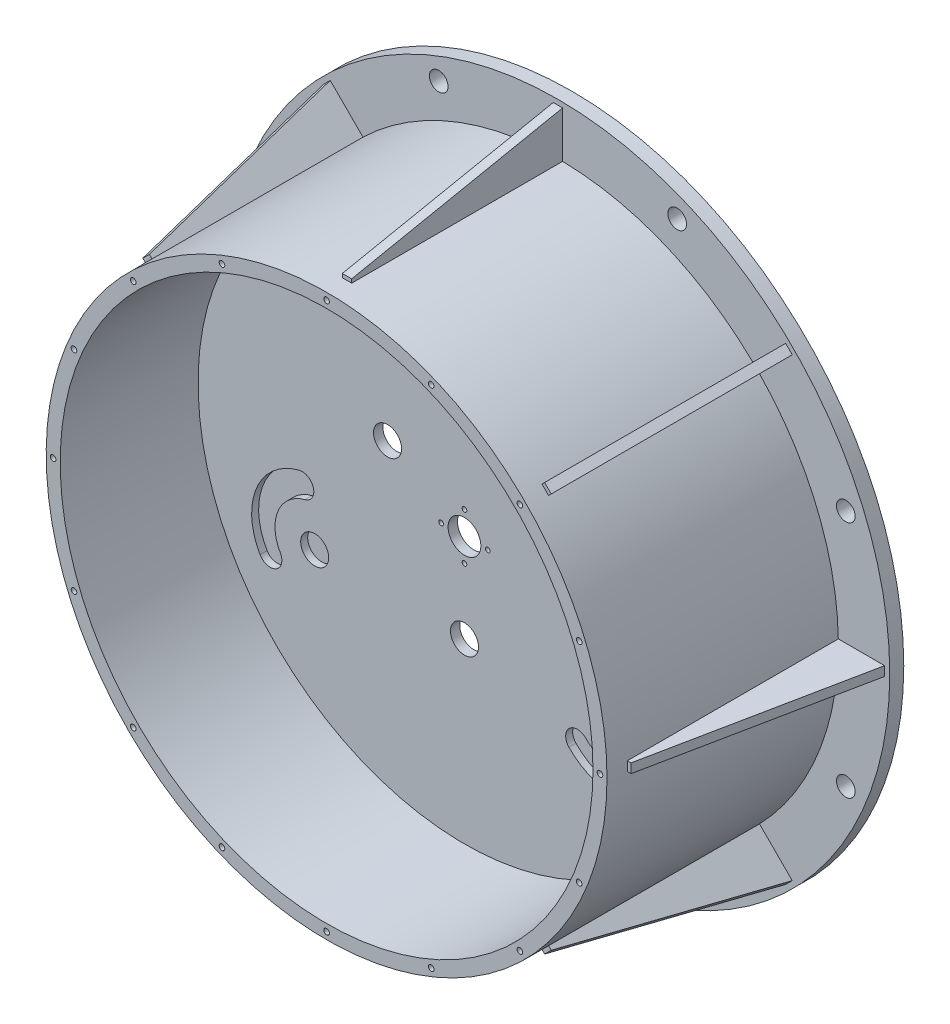
SolidWorks part; units mm, degrees
ref_plane "Front Plane" through (0, 0, 0) normal (0, 0, 1) x (1, 0, 0)
ref_plane "Top Plane" through (0, 0, 0) normal (0, 1, 0) x (1, 0, 0)
ref_plane "Right Plane" through (0, 0, 0) normal (1, 0, 0) x (0, 0, -1)
sketch "Sketch1" plane through (0, 0, 0) normal (0, 0, 1) x (1, 0, 0)
  circle A0 centre (0, 0) radius 600
  dimension "D1" = 1200
extrude "Boss-Extrude1" add sketch "Sketch1" along normal blind 20
sketch "Sketch2" plane through (0, 0, 0) normal (0, 0, -1) x (-1, 0, 0)
  circle A0 centre (0, 0) radius 35
  circle A1 centre (0, 0) radius 50 construction
  circle A2 centre (50, 0) radius 5
  circle A3 centre (0, -50) radius 5
  circle A4 centre (-50, 0) radius 5
  circle A5 centre (0, 50) radius 5
  point P15 (0, 0)
  dimension "D1" = 70
  dimension "D2" = 100
  dimension "D3" = 10
  dimension "D4" = 4
extrude "Cut-Extrude1" cut sketch "Sketch2" against normal through all
sketch "Sketch3" plane through (0, 0, 0) normal (0, 0, -1) x (-1, 0, 0)
  line L0 (0, 0) -> (0, -190) construction
  circle A0 centre (0, -190) radius 30
  dimension "D2" = 60
  dimension "D1" = 190
extrude "Cut-Extrude2" cut sketch "Sketch3" against normal through all
pattern_circular "CirPattern1" count 3 over 360 about axis through (0, 0, 0) along (0, 0, 1) of "Cut-Extrude2"
sketch "Sketch4" plane through (0, 0, 20) normal (0, 0, 1) x (1, 0, 0)
  circle A0 centre (0, 0) radius 600
  circle A1 centre (0, 0) radius 570
  dimension "D1" = 30
  dimension "D2" = 1200
extrude "Boss-Extrude2" add sketch "Sketch4" against normal blind 200
sketch "Sketch6" plane through (0, 0, 20) normal (0, 0, 1) x (1, 0, 0)
  line L0 (0, 0) -> (0, 550) construction
  circle A2 centre (0, 370) radius 30
  circle A3 centre (320.4294, -185) radius 30
  circle A4 centre (-320.4294, -185) radius 30
  arc A5 (96.3228, 316.8783) -> (-24.8381, 477.1591) centre (0, 370) ccw construction
  arc A10 (437.3428, -252.5) -> (394.0416, -227.5) centre (415.6922, -240) ccw
  arc A11 (259.4645, -244.2307) -> (394.0416, -227.5) centre (320.4294, -185) ccw
  arc A12 (259.4645, -244.2307) -> (223.6028, -279.0723) centre (241.5336, -261.6515) ccw
  arc A13 (223.6028, -279.0723) -> (437.3428, -252.5) centre (320.4294, -185) ccw
  arc A14 (-437.3428, -252.5) -> (-394.0416, -227.5) centre (-415.6922, -240) ccw
  arc A15 (-341.2422, -102.5875) -> (-394.0416, -227.5) centre (-320.4294, -185) ccw
  arc A16 (-341.2422, -102.5875) -> (-353.4851, -54.1095) centre (-347.3637, -78.3485) ccw
  arc A17 (-353.4851, -54.1095) -> (-437.3428, -252.5) centre (-320.4294, -185) ccw
  arc A30 (81.7778, 346.8182) -> (0, 455) centre (0, 370) ccw
  arc A31 (0, 505) -> (0, 455) centre (0, 480) ccw
  arc A32 (129.8823, 333.1818) -> (0, 505) centre (0, 370) ccw
  arc A33 (81.7778, 346.8182) -> (129.8823, 333.1818) centre (105.8301, 340) ccw
  point P11 (0, 0)
  point P37 (0, 0)
  dimension "D1" = 60
  dimension "D2" = 60
  dimension "D4" = 60
  dimension "D5" = 220
extrude "Cut-Extrude3" cut sketch "Sketch6" against normal blind 15
sketch "Sketch7" plane through (0, 0, 20) normal (0, 0, 1) x (1, 0, 0)
  circle A0 centre (0, 0) radius 600
  circle A1 centre (0, 0) radius 570
  dimension "D1" = 1200
  dimension "D2" = 30
extrude "Boss-Extrude3" add sketch "Sketch7" along normal blind 295
sketch "Sketch8" plane through (0, 0, -180) normal (0, 0, -1) x (-1, 0, 0)
  line L0 (0, 0) -> (710, 0) construction
  line L1 (0, 0) -> (615.9803, -255.1474) construction
  circle A0 centre (0, 0) radius 570
  circle A1 centre (0, 0) radius 710
  circle A2 centre (-615.9803, 255.1474) radius 20
  circle A3 centre (-255.1474, 615.9803) radius 20
  circle A4 centre (255.1474, 615.9803) radius 20
  circle A5 centre (615.9803, 255.1474) radius 20
  circle A6 centre (615.9803, -255.1474) radius 20
  circle A7 centre (255.1474, -615.9803) radius 20
  circle A8 centre (-255.1474, -615.9803) radius 20
  circle A9 centre (-615.9803, -255.1474) radius 20
  point P23 (0, 0)
  dimension "D1" = 1420
  dimension "D2" = 40
  dimension "D5" = 1140
  dimension "D4" = 22.5
  dimension "D3" = 8
extrude "Boss-Extrude4" add sketch "Sketch8" along normal blind 30
sketch "Sketch9" plane through (0, 0, 315) normal (0, 0, 1) x (1, 0, 0)
  circle A0 centre (0, 0) radius 585 construction
  circle A1 centre (585, 0) radius 6
  circle A2 centre (540.4695, -223.8698) radius 6
  circle A3 centre (413.6575, -413.6575) radius 6
  circle A4 centre (223.8698, -540.4695) radius 6
  circle A5 centre (0, -585) radius 6
  circle A6 centre (-223.8698, -540.4695) radius 6
  circle A7 centre (-413.6575, -413.6575) radius 6
  circle A8 centre (-540.4695, -223.8698) radius 6
  circle A9 centre (-585, 0) radius 6
  circle A10 centre (-540.4695, 223.8698) radius 6
  circle A11 centre (-413.6575, 413.6575) radius 6
  circle A12 centre (-223.8698, 540.4695) radius 6
  circle A13 centre (0, 585) radius 6
  circle A14 centre (223.8698, 540.4695) radius 6
  circle A15 centre (413.6575, 413.6575) radius 6
  circle A16 centre (540.4695, 223.8698) radius 6
  point P38 (0, 0)
  dimension "D1" = 12
  dimension "D3" = 1170
  dimension "D2" = 16
extrude "Cut-Extrude4" cut sketch "Sketch9" against normal blind 30
sketch "Sketch10" plane through (0, 0, 0) normal (0, 1, 0) x (1, 0, 0)
  line L1 (-600, 180) -> (600, 180) construction
  line L2 (-594.3176, 180) -> (-594.3176, -271.3296)
  line L4 (-607.9361, -271.3296) -> (-698.9937, 180)
  line L5 (-710, 180) -> (710, 180) construction
  line L6 (-698.9937, 180) -> (-594.3176, 180)
  line L7 (-594.3176, -271.3296) -> (-607.9361, -271.3296)
extrude "Boss-Extrude5" add sketch "Sketch10" along normal mid plane 20
pattern_circular "CirPattern2" count 8 over 360 about axis through (0, 0, 0) along (0, 0, 1) of "Boss-Extrude5"
equation "\"A\"= \"代号代码\""
equation "\"B\"= \"名称代码\""
